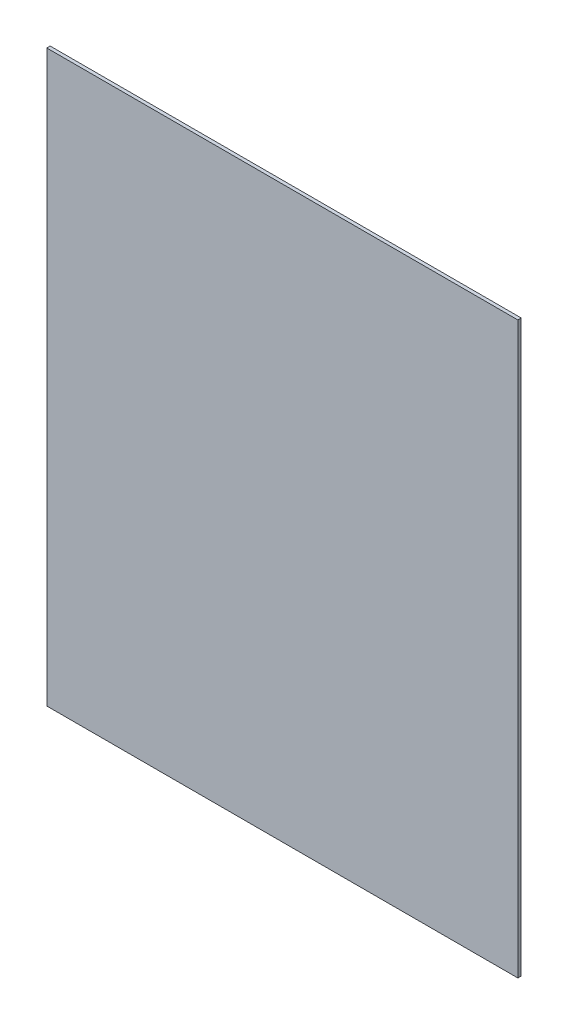
from build123d import *

# Parameters (mm, degrees)
SKETCH_1_W      = 696
SKETCH_1_H      = 842
EXTRUDE_1_DEPTH = 5


with BuildPart() as part:
    # 草图1 → 凸台-拉伸1 (new body)
    with BuildSketch(Plane.XY):
        Rectangle(SKETCH_1_W, SKETCH_1_H)
    extrude(amount=EXTRUDE_1_DEPTH)


solid = part.part
